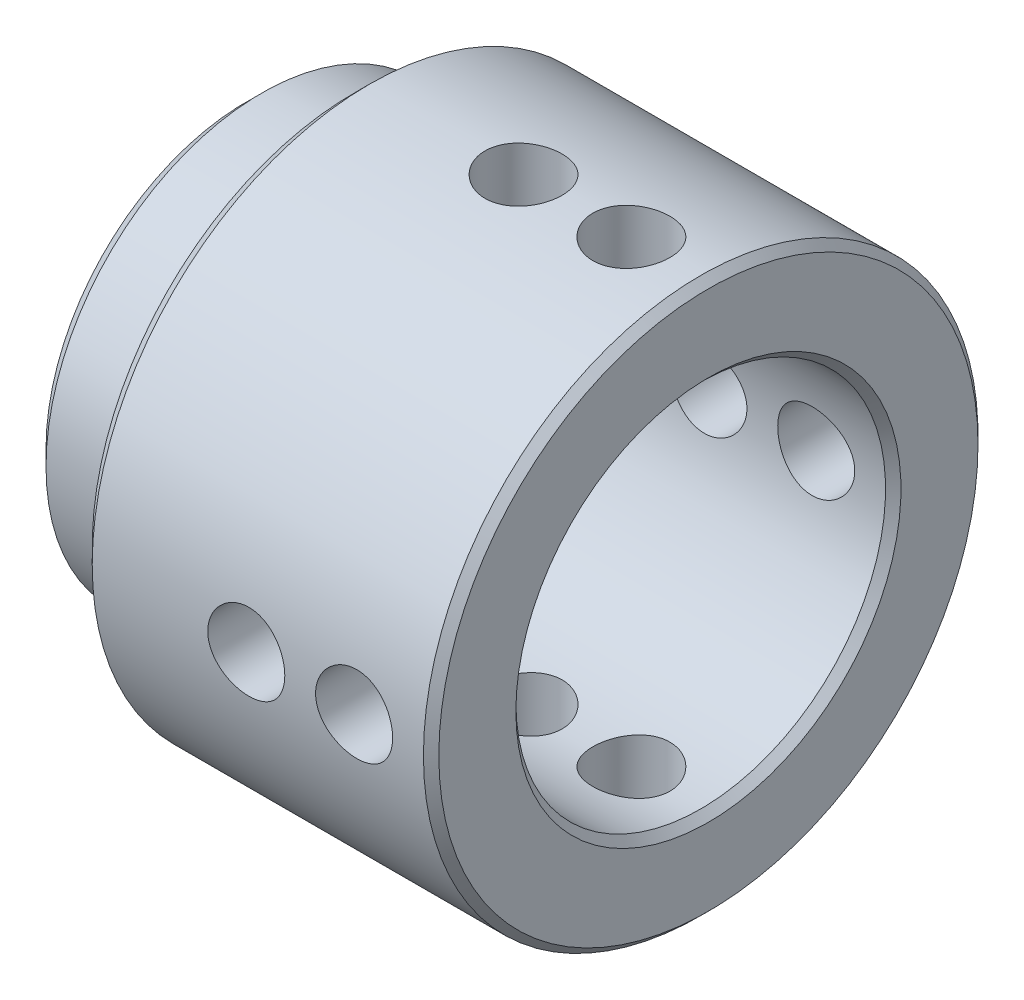
SolidWorks part; units mm, degrees
ref_plane "前视基准面" through (0, 0, 0) normal (0, 0, 1) x (1, 0, 0)
ref_plane "上视基准面" through (0, 0, 0) normal (0, 1, 0) x (1, 0, 0)
ref_plane "右视基准面" through (0, 0, 0) normal (1, 0, 0) x (0, 0, -1)
sketch "草图1" plane through (0, 0, 0) normal (0, 0, 1) x (1, 0, 0)
  line L0 (0, 0) -> (20.5578, 0) construction
  line L1 (0, 5) -> (12, 5)
  line L2 (12, 5) -> (12, 12)
  line L3 (12, 12) -> (30, 12)
  line L4 (30, 12) -> (30, 18)
  line L5 (30, 18) -> (7, 18)
  line L6 (7, 18) -> (7, 14)
  line L7 (7, 14) -> (0, 14)
  line L8 (0, 14) -> (0, 5)
  dimension "D1" = 5
  dimension "D2" = 12
  dimension "D3" = 7
  dimension "D4" = 6
  dimension "D5" = 18
  dimension "D6" = 23
  dimension "D7" = 4
revolve "旋转1" add sketch "草图1" angle 360 about L0
sketch "草图2" plane through (0, 0, 0) normal (-1, 0, 0) x (0, 0, 1)
  line L1 (-2, 0) -> (2, 0)
  line L2 (-2, 0) -> (-2, 6.5)
  line L3 (-2, 6.5) -> (2, 6.5)
  line L4 (2, 0) -> (2, 6.5)
  dimension "D1" = 6.5
  dimension "D2" = 4
  dimension "D3" = 2
extrude "切除-拉伸1" cut sketch "草图2" against normal through all
sketch "草图3" plane through (0, 0, 0) normal (0, 1, 0) x (1, 0, 0)
  line L0 (30, -18) -> (30, 18) construction
  circle A0 centre (18, 0) radius 2.5
  circle A1 centre (25, 0) radius 2.5
  dimension "D1" = 5
  dimension "D2" = 5
  dimension "D3" = 5
  dimension "D4" = 12
extrude "切除-拉伸2" cut sketch "草图3" against normal through all and the other way through all
chamfer "倒角1" distance 1 angle 45 2 edges at (7, 0, 18) (0, 0, 14)
chamfer "倒角2" distance 0.5 angle 45 2 edges at (30, 0, 12) (30, 0, 18)
sketch "草图4" plane through (0, 0, 0) normal (0, 0, 1) x (1, 0, 0)
  line L0 (30, -17.5) -> (30, 17.5) construction
  circle A0 centre (25, 0) radius 2.5
  circle A1 centre (18, 0) radius 2.5
  dimension "D1" = 5
  dimension "D2" = 5
  dimension "D3" = 5
  dimension "D4" = 12
extrude "切除-拉伸3" cut sketch "草图4" against normal through all and the other way through all
